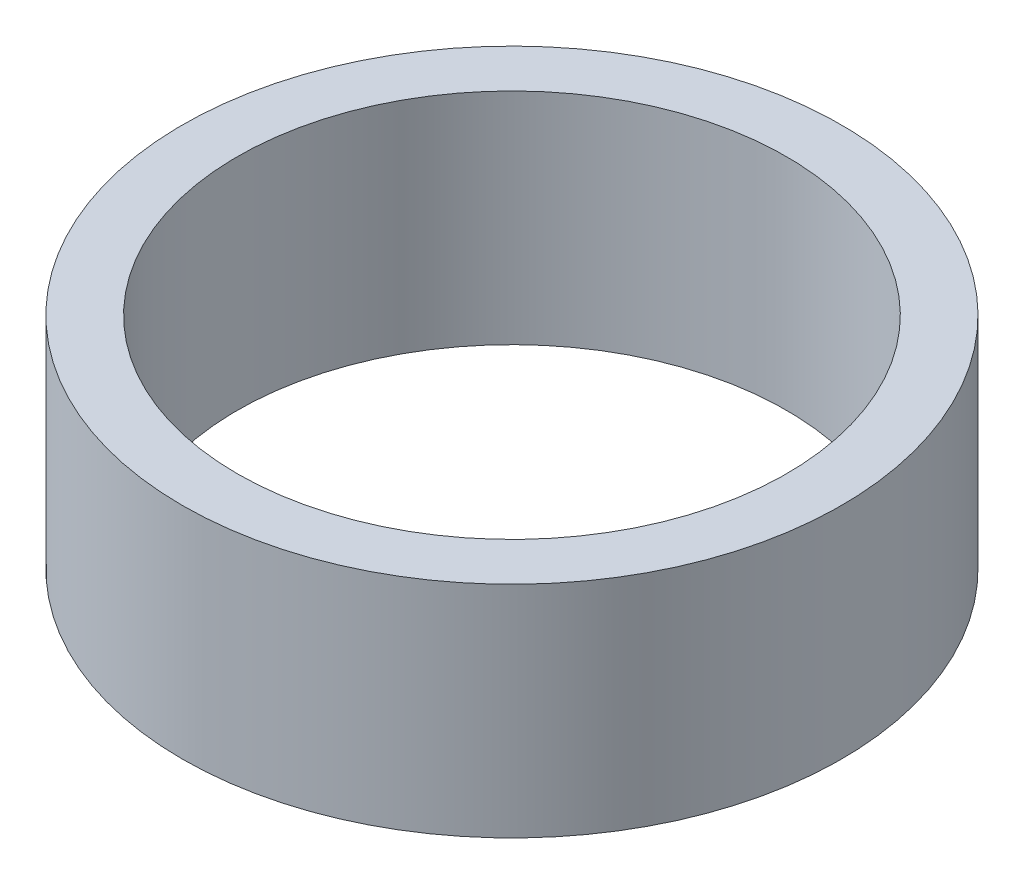
SolidWorks part; units mm, degrees
ref_plane "Front Plane" through (0, 0, 0) normal (0, 0, 1) x (1, 0, 0)
ref_plane "Top Plane" through (0, 0, 0) normal (0, 1, 0) x (1, 0, 0)
ref_plane "Right Plane" through (0, 0, 0) normal (1, 0, 0) x (0, 0, -1)
other "Configuration Table"
sketch "Sketch1" plane through (0, 0, 0) normal (0, 1, 0) x (1, 0, 0)
  circle A0 centre (0, 0) radius 3
  circle A1 centre (0, 0) radius 2.5
  dimension "D1" = 6
  dimension "D2" = 5
extrude "Boss-Extrude1" add sketch "Sketch1" along normal blind 2
